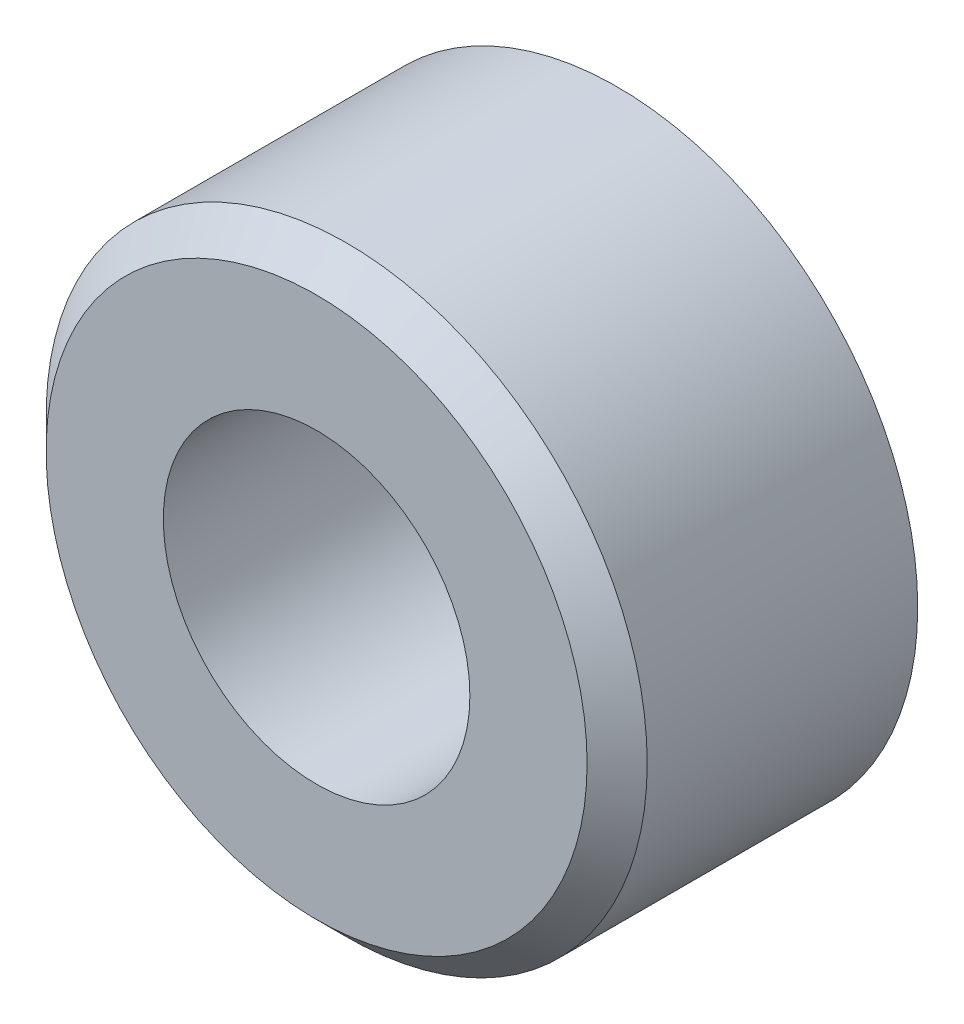
SolidWorks part; units mm, degrees
material "1023 碳钢板 (SS)"
ref_plane "前视基准面" through (0, 0, 0) normal (0, 0, 1) x (1, 0, 0)
ref_plane "上视基准面" through (0, 0, 0) normal (0, 1, 0) x (1, 0, 0)
ref_plane "右视基准面" through (0, 0, 0) normal (1, 0, 0) x (0, 0, -1)
sketch "草图1" plane through (0, 0, 0) normal (0, 0, 1) x (1, 0, 0)
  circle A0 centre (0, 0) radius 10
  dimension "D1" = 20
extrude "凸台-拉伸1" add sketch "草图1" along normal blind 10
hole_wizard "M12 螺纹孔1" positions "草图2" profile "草图3" tap size "M12" standard "GB"
sketch "草图2" plane through (0, 0, 10) normal (0, 0, 1) x (1, 0, 0)
  point P0 (0, 0)
sketch "草图3" plane through (0, 0, 10) normal (1, 0, 0) x (0, -1, 0)
  line L0 (0, 0) -> (0, 33.3144)
  line L1 (0, 33.3144) -> (5.1, 30.25)
  line L2 (5.1, 30.25) -> (5.1, 0)
  line L5 (5.1, 0) -> (0, 0)
  line L10 (0, 33.3144) -> (-5.1, 30.25) construction
  line L11 (0, -6.35) -> (0, 107.95) construction
  dimension "螺纹孔钻头直径" = 10.2
  dimension "螺纹孔钻头深度" = 30.25
  dimension "导头角度" = 118
cosmetic thread "孔螺蚊线1"
chamfer "倒角1" distance 1 angle 45 1 edges at (10, 0, 10)
